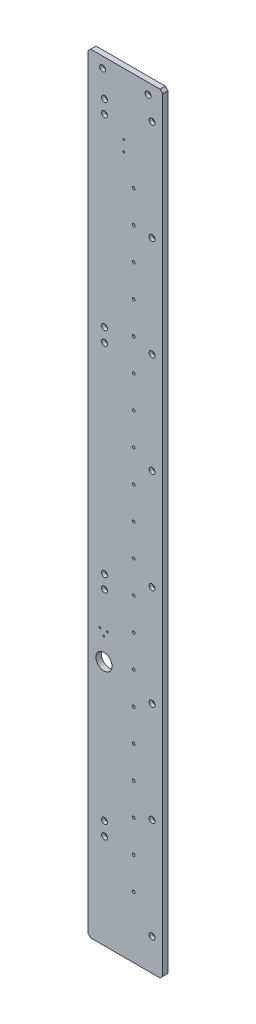
from build123d import *

# Parameters (mm, degrees)
SKETCH_1_W                     = 140
SKETCH_1_H                     = 1440
EXTRUDE_1_DEPTH                = 10
HOLE_WIZARD_M6_1_D             = 5
HOLE_WIZARD_M6_1_2_D           = 6.6
HOLE_WIZARD_M6_1_2_DEPTH       = 17
HOLE_WIZARD_M6_1_2_CBORE_D     = 11
HOLE_WIZARD_M6_1_2_CBORE_DEPTH = 6.4
HOLE_WIZARD_M6_1_2_TIP         = 1.982840043
HOLE_WIZARD_M4_1_D             = 3.3
SKETCH_9_R                     = 15
CUT_EXTRUDE_2_DEPTH            = 10
CHAMFER_1_SIZE                 = 5
HOLE_WIZARD_M6_2_D             = 6.6
HOLE_WIZARD_M6_2_DEPTH         = 17
HOLE_WIZARD_M6_2_CBORE_D       = 11
HOLE_WIZARD_M6_2_CBORE_DEPTH   = 6.4
HOLE_WIZARD_M6_2_TIP           = 1.982840043
HOLE_WIZARD_M4_2_D             = 3.3
HOLE_WIZARD_M4_2_DEPTH         = 11.5
HOLE_WIZARD_M4_2_TIP           = 0.991420021


with BuildPart() as part:
    # 草图1 → 凸台-拉伸1 (new body)
    with BuildSketch(Plane.XY):
        with Locations((70, -720)):
            Rectangle(SKETCH_1_W, SKETCH_1_H)
    extrude(amount=EXTRUDE_1_DEPTH)

    # Hole Wizard M6 _1 (through all)
    with Locations(Plane.XY.offset(10)):
        with Locations((85.75, -185), (85.75, -245), (85.75, -305), (85.75, -365), (85.75, -425), (85.75, -485), (85.75, -545), (85.75, -605), (85.75, -665), (85.75, -725), (85.75, -785), (85.75, -845), (85.75, -905), (85.75, -965), (85.75, -1025), (85.75, -1085), (85.75, -1145), (85.75, -1205), (85.75, -1265), (85.75, -1325)):
            Hole(HOLE_WIZARD_M6_1_D / 2)

    # Hole Wizard M6 _1 2
    with Locations(Plane.XY.offset(10)):
        with Locations((31, -1262.5), (31, -1237.5), (31, -862.5), (31, -837.5), (31, -462.5), (31, -437.5), (31, -92.5), (31, -67.5)):
            CounterBoreHole(HOLE_WIZARD_M6_1_2_D / 2, HOLE_WIZARD_M6_1_2_CBORE_D / 2, HOLE_WIZARD_M6_1_2_CBORE_DEPTH, depth=HOLE_WIZARD_M6_1_2_DEPTH)
            with Locations((0, 0, -(HOLE_WIZARD_M6_1_2_DEPTH + HOLE_WIZARD_M6_1_2_TIP / 2))):  # 118° drill point
                Cone(0, HOLE_WIZARD_M6_1_2_D / 2, HOLE_WIZARD_M6_1_2_TIP, mode=Mode.SUBTRACT)

    # M4 螺纹孔1 (through all)
    with Locations(Plane.XY.offset(10)):
        with Locations((22.5, -928.5), (36.5, -928.5), (29.5, -938.5)):
            Hole(HOLE_WIZARD_M4_1_D / 2)

    # 草图9 → 切除-拉伸2 (cut)
    with BuildSketch(Plane.XY.offset(10)):
        with Locations((30, -980)):
            Circle(SKETCH_9_R)
    extrude(amount=-CUT_EXTRUDE_2_DEPTH, mode=Mode.SUBTRACT)

    # 倒角1
    chamfer_1_edges = [part.edges().sort_by_distance(p)[0] for p in [
        (0, 0, 5),
        (140, 0, 5),
        (140, -1440, 5),
        (0, -1440, 5),
    ]]
    chamfer(chamfer_1_edges, length=CHAMFER_1_SIZE)

    # M6 六角凹头螺钉的柱形沉头孔2
    with Locations(Plane.XY.offset(10)):
        with Locations((120, -1380), (120, -1191.428571429), (120, -1002.857142857), (120, -814.285714286), (120, -625.714285714), (120, -437.142857143), (120, -248.571428571), (120, -60), (27.5, -20), (112.5, -20)):
            CounterBoreHole(HOLE_WIZARD_M6_2_D / 2, HOLE_WIZARD_M6_2_CBORE_D / 2, HOLE_WIZARD_M6_2_CBORE_DEPTH, depth=HOLE_WIZARD_M6_2_DEPTH)
            with Locations((0, 0, -(HOLE_WIZARD_M6_2_DEPTH + HOLE_WIZARD_M6_2_TIP / 2))):  # 118° drill point
                Cone(0, HOLE_WIZARD_M6_2_D / 2, HOLE_WIZARD_M6_2_TIP, mode=Mode.SUBTRACT)

    # M4 螺纹孔2
    with Locations(Plane.XY.offset(10)):
        with Locations((67, -115.5), (67, -135.5)):
            Hole(HOLE_WIZARD_M4_2_D / 2, depth=HOLE_WIZARD_M4_2_DEPTH)
            with Locations((0, 0, -(HOLE_WIZARD_M4_2_DEPTH + HOLE_WIZARD_M4_2_TIP / 2))):  # 118° drill point
                Cone(0, HOLE_WIZARD_M4_2_D / 2, HOLE_WIZARD_M4_2_TIP, mode=Mode.SUBTRACT)


solid = part.part
